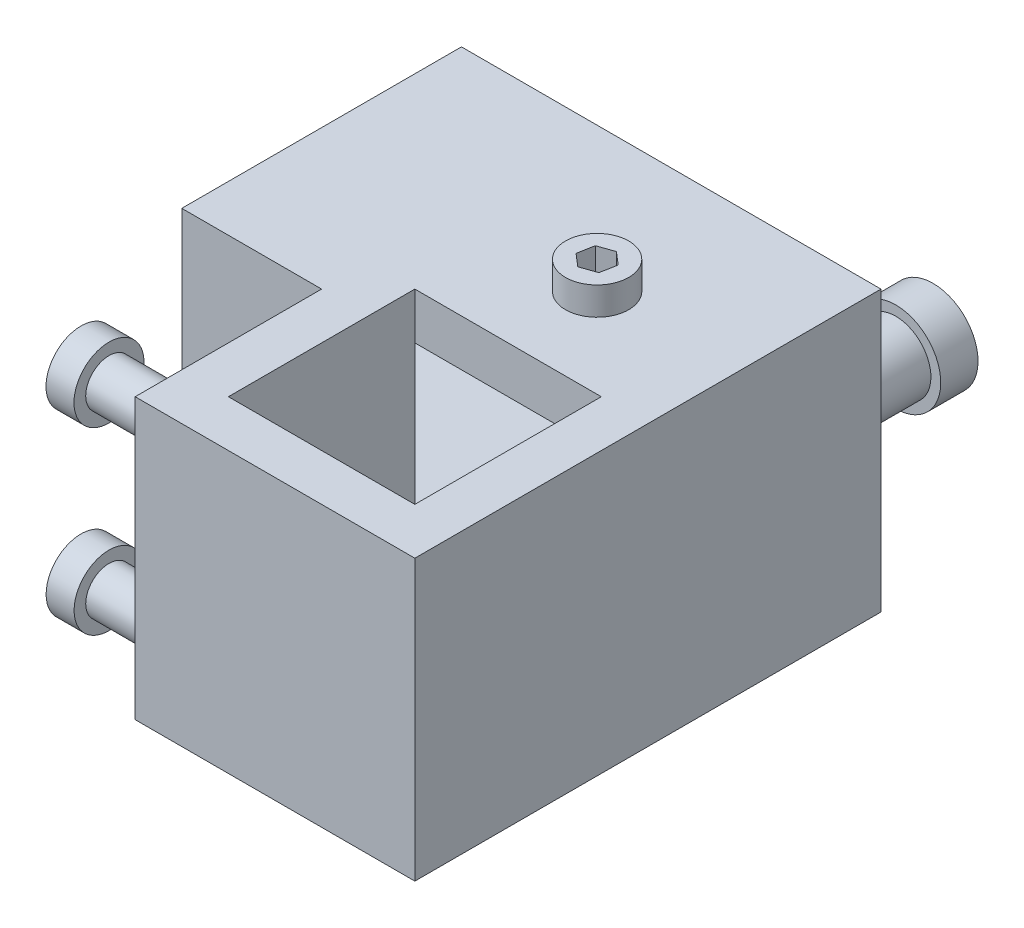
from build123d import *

# Parameters (mm, degrees)
SKETCH1_W                = 60
SKETCH1_H                = 60
SKETCH1_W_2              = 40
SKETCH1_H_2              = 40
BOSS_EXTRUDE1_DEPTH      = 60
BOSS_EXTRUDE2_DEPTH      = 30
BOSS_EXTRUDE2_DEPTH_BACK = 60
CUT_EXTRUDE1_DEPTH       = 50
CUT_EXTRUDE1_DEPTH_BACK  = 50
SKETCH3_W                = 40
SKETCH3_H                = 40
SKETCH4_W                = 40
SKETCH4_H                = 10
CUT_EXTRUDE2_DEPTH       = 60
SKETCH5_R                = 9.65079084
BOSS_EXTRUDE3_DEPTH      = 4
SKETCH6_R                = 7.543593384
BOSS_EXTRUDE4_DEPTH      = 15
SKETCH7_R                = 9.65079084
BOSS_EXTRUDE5_DEPTH      = 8
SKETCH8_R                = 3
CUT_EXTRUDE3_DEPTH       = 18
SKETCH9_R                = 3.727144442
SKETCH9_R_2              = 3.681065336
BOSS_EXTRUDE6_DEPTH      = 4
SKETCH10_R               = 6.781063786
BOSS_EXTRUDE7_DEPTH      = 6
SKETCH11_R               = 6.541743029
BOSS_EXTRUDE8_DEPTH      = 6
SKETCH12_R               = 5
BOSS_EXTRUDE9_DEPTH      = 16
SKETCH13_R               = 7.492042748
SKETCH13_R_2             = 7.517434031
BOSS_EXTRUDE10_DEPTH     = 6


with BuildPart() as part:
    # Sketch1 → Boss-Extrude1 (new body)
    with BuildSketch(Plane(origin=(0, 0, 0), x_dir=(1, 0, 0), z_dir=(0, 1, 0))):
        Rectangle(SKETCH1_W, SKETCH1_H)
        Rectangle(SKETCH1_W_2, SKETCH1_H_2, mode=Mode.SUBTRACT)
    extrude(amount=BOSS_EXTRUDE1_DEPTH)

    # Sketch2 → Boss-Extrude2 (add, two sides: drawn at the far end of the back side and taken through both)
    with BuildSketch(Plane.ZY.offset(30).offset(-BOSS_EXTRUDE2_DEPTH_BACK)):
        Polygon((-30, 60), (-70, 60), (-70, 0), (-30, 0), (-10, 0), (-10, 60), align=None)
    extrude(amount=BOSS_EXTRUDE2_DEPTH + BOSS_EXTRUDE2_DEPTH_BACK)

    # Sketch3 → Cut-Extrude1 (cut, two sides: drawn at the far end of the back side and taken through both)
    with BuildSketch(Plane.ZY.offset(30).offset(-CUT_EXTRUDE1_DEPTH_BACK)):
        with Locations((-40, 30)):
            Rectangle(SKETCH3_W, SKETCH3_H)
    extrude(amount=CUT_EXTRUDE1_DEPTH + CUT_EXTRUDE1_DEPTH_BACK, mode=Mode.SUBTRACT)

    # Sketch4 → Cut-Extrude2 (cut)
    with BuildSketch(Plane(origin=(0, 60, 0), x_dir=(1, 0, 0), z_dir=(0, 1, 0))):
        with Locations((0, 15)):
            Rectangle(SKETCH4_W, SKETCH4_H)
    extrude(amount=-CUT_EXTRUDE2_DEPTH, mode=Mode.SUBTRACT)

    # Sketch5 → Boss-Extrude3 (add)
    with BuildSketch(Plane(origin=(0, 0, -70), x_dir=(-1, 0, 0), z_dir=(0, 0, -1))):
        with Locations(Location((-14.164480052, 30, 0), (0, 0, 270))):
            Circle(SKETCH5_R)
    extrude(amount=BOSS_EXTRUDE3_DEPTH)

    # Sketch6 → Boss-Extrude4 (add)
    with BuildSketch(Plane(origin=(0, 0, -74), x_dir=(-1, 0, 0), z_dir=(0, 0, -1))):
        with Locations(Location((-14.164480052, 30, 0), (0, 0, 90))):
            Circle(SKETCH6_R)
    extrude(amount=BOSS_EXTRUDE4_DEPTH)

    # Sketch7 → Boss-Extrude5 (add)
    with BuildSketch(Plane(origin=(0, 0, -89), x_dir=(-1, 0, 0), z_dir=(0, 0, -1))):
        with Locations(Location((-14.164480052, 30, 0), (0, 0, 270))):
            Circle(SKETCH7_R)
    extrude(amount=BOSS_EXTRUDE5_DEPTH)

    # Sketch8 → Cut-Extrude3 (cut)
    with BuildSketch(Plane(origin=(0, 0, -70), x_dir=(-1, 0, 0), z_dir=(0, 0, -1))):
        with Locations(Location((13.782784639, 47, 0), (0, 0, 90))):
            Circle(SKETCH8_R)
        with Locations(Location((13.782784639, 13, 0), (0, 0, 90))):
            Circle(SKETCH8_R)
    extrude(amount=-CUT_EXTRUDE3_DEPTH, mode=Mode.SUBTRACT)

    # Sketch9 → Boss-Extrude6 (add)
    # profile 1 of 2: a face of its own
    with BuildSketch(Plane(origin=(0, 0, -70), x_dir=(-1, 0, 0), z_dir=(0, 0, -1))):
        with Locations(Location((46.11202463, 47.187080899, 0), (0, 0, 270))):
            Circle(SKETCH9_R)
        Polygon((47.572683063, 45.726422466), (48.107321156, 47.721718992), (46.646662723, 49.182377425), (44.651366197, 48.647739332), (44.116728104, 46.652442806), (45.577386537, 45.191784373), align=None, mode=Mode.SUBTRACT)
    # profile 2 of 2: a face of its own
    with BuildSketch(Plane(origin=(0, 0, -70), x_dir=(-1, 0, 0), z_dir=(0, 0, -1))):
        with Locations(Location((46.11202463, 12.520787414, 0), (0, 0, 270))):
            Circle(SKETCH9_R_2)
        Polygon((47.572683063, 11.352260668), (47.854327694, 13.201491351), (46.393669261, 14.370018097), (44.651366197, 13.689314161), (44.369721566, 11.840083478), (45.830379999, 10.671556732), align=None, mode=Mode.SUBTRACT)
    extrude(amount=BOSS_EXTRUDE6_DEPTH)

    # Sketch10 → Boss-Extrude7 (add)
    with BuildSketch(Plane(origin=(0, 60, 0), x_dir=(1, 0, 0), z_dir=(0, 1, 0))):
        with Locations(Location((0, 39.10148189, 0), (0, 0, 270))):
            Circle(SKETCH10_R)
        Polygon((2.69356978, 36.789759205), (3.348795461, 40.278320404), (0.655225682, 42.590043088), (-2.69356978, 41.413204575), (-3.348795461, 37.924643376), (-0.655225682, 35.612920692), align=None, mode=Mode.SUBTRACT)
    extrude(amount=BOSS_EXTRUDE7_DEPTH)

    # Sketch11 → Boss-Extrude8 (add)
    with BuildSketch(Plane.XZ):
        with Locations(Location((0, -37.145408849, 0), (0, 0, 90))):
            Circle(SKETCH11_R)
        Polygon((2.337920136, -39.990606), (3.632973079, -36.543309195), (1.295052943, -33.698112044), (-2.337920136, -34.300211699), (-3.632973079, -37.747508503), (-1.295052943, -40.592705654), align=None, mode=Mode.SUBTRACT)
    extrude(amount=BOSS_EXTRUDE8_DEPTH)

    # Sketch12 → Boss-Extrude9 (add)
    with BuildSketch(Plane.ZY.offset(30)):
        with Locations(Location((19.608999651, 49.443527686, 0), (0, 0, 180))):
            Circle(SKETCH12_R)
        with Locations(Location((19.608999651, 10.831292493, 0), (0, 0, 180))):
            Circle(SKETCH12_R)
    extrude(amount=BOSS_EXTRUDE9_DEPTH)

    # Sketch13 → Boss-Extrude10 (add)
    # profile 1 of 2: a face of its own
    with BuildSketch(Plane.ZY.offset(46)):
        with Locations((19.608999651, 10.831292493)):
            Circle(SKETCH13_R)
        Polygon((22.246303592, 7.024085978), (24.224789181, 11.211661446), (21.58748524, 15.018867961), (16.971695711, 14.638499008), (14.993210122, 10.45092354), (17.630514063, 6.643717026), align=None, mode=Mode.SUBTRACT)
    # profile 2 of 2: a face of its own
    with BuildSketch(Plane.ZY.offset(46)):
        with Locations((19.608999651, 49.443527686)):
            Circle(SKETCH13_R_2)
        Polygon((22.809739777, 46.848480214), (23.456746749, 50.91792621), (20.256006623, 53.512973682), (16.408259526, 52.038575158), (15.761252554, 47.969129162), (18.96199268, 45.37408169), align=None, mode=Mode.SUBTRACT)
    extrude(amount=BOSS_EXTRUDE10_DEPTH)


solid = part.part
